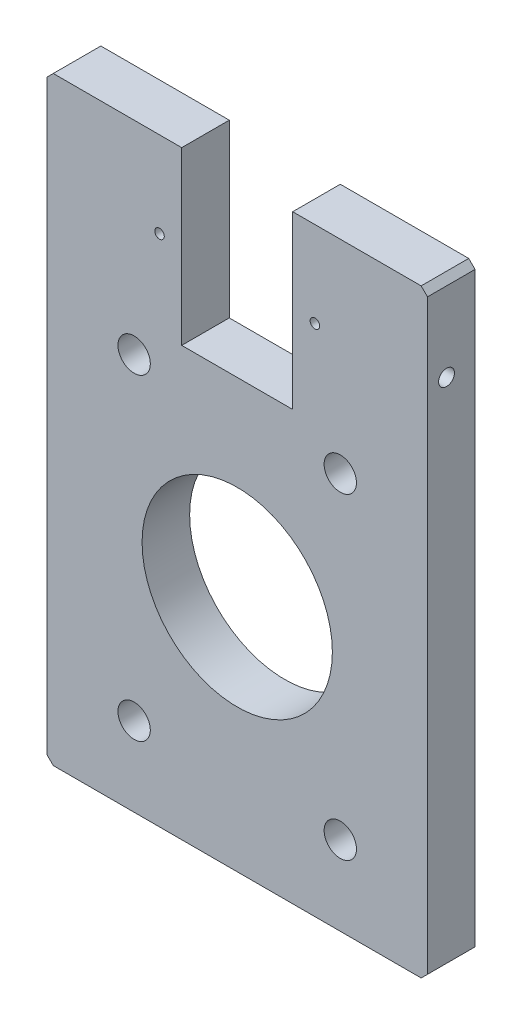
SolidWorks part; units mm, degrees
material "1023 碳钢板 (SS)"
ref_plane "Front Plane" through (0, 0, 0) normal (0, 0, 1) x (1, 0, 0)
ref_plane "Top Plane" through (0, 0, 0) normal (0, 1, 0) x (1, 0, 0)
ref_plane "Right Plane" through (0, 0, 0) normal (1, 0, 0) x (0, 0, -1)
sketch "Sketch1" plane through (0, 0, 0) normal (0, 0, 1) x (1, 0, 0)
  line L0 (17.5, 94.5) -> (58, 94.5)
  line L1 (-58, 94.5) -> (-17.5, 94.5)
  line L2 (-60, 92.5) -> (-60, -92.5)
  line L3 (-58, -94.5) -> (58, -94.5)
  line L4 (60, 92.5) -> (60, -92.5)
  line L5 (-60, 94.5) -> (60, -94.5) construction
  line L6 (-60, -94.5) -> (60, 94.5) construction
  line L8 (-17.5, 94.5) -> (-17.5, 40.5)
  line L9 (-17.5, 40.5) -> (17.5, 40.5)
  line L10 (17.5, 94.5) -> (17.5, 40.5)
  line L11 (-17.5, 148.5) -> (17.5, 40.5) construction
  line L12 (-17.5, 40.5) -> (17.5, 148.5) construction
  line L13 (-60, 92.5) -> (-58, 94.5)
  line L14 (58, 94.5) -> (60, 92.5)
  line L15 (-60, -92.5) -> (-58, -94.5)
  line L16 (58, -94.5) -> (60, -92.5)
  circle A0 centre (-32.5, -69.5) radius 5.1
  circle A1 centre (-32.5, 30.5) radius 5.1
  circle A2 centre (32.5, 30.5) radius 5.1
  circle A3 centre (32.5, -69.5) radius 5.1
  point P0 (0, 0)
  point P6 (0, 94.5)
  point P23 (0, -94.5)
  dimension "D13" = 32.5
  dimension "D15" = 10.2
  dimension "D16" = 65
  dimension "D1" = 120
  dimension "D2" = 189
  dimension "D3" = 35
  dimension "D4" = 108
  dimension "D5" = 2
  dimension "D6" = 45
  dimension "D7" = 2
  dimension "D8" = 45
  dimension "D9" = 2
  dimension "D10" = 45
  dimension "D11" = 2
  dimension "D12" = 45
  dimension "D14" = 25
  dimension "D17" = 100
  dimension "D18" = 100
  dimension "D19" = 65
extrude "Boss-Extrude1" add sketch "Sketch1" along normal blind 15
hole_wizard "Size mm dowel hole 1" positions "3DSketch6" profile "Sketch20" hole size "Ø3.0" standard "IS"
sketch3d "3DSketch6"
  point P0 (60, 67.5, 9)
  dimension "D1" = 9
  dimension "D2" = 27
sketch "Sketch20" plane through (60, 67.5, 9) normal (0, 1, 0) x (0, 0, -1)
  line L0 (0, 0) -> (0, 40)
  line L1 (0, 40) -> (1.5, 39.0987)
  line L2 (1.5, 39.0987) -> (1.5, 0)
  line L5 (1.5, 0) -> (0, 0)
  line L10 (0, 40) -> (-1.5, 39.0987) construction
  line L11 (0, -6.35) -> (0, 107.95) construction
  dimension "孔直径" = 3
  dimension "孔深度" = 40
  dimension "导头角度" = 118
hole_wizard "Size mm dowel hole 2" positions "3DSketch7" profile "Sketch21" hole size "Ø3.0" standard "IS"
sketch3d "3DSketch7"
  point P0 (-60, 67.5, 9)
  dimension "D1" = 27
  dimension "D2" = 9
sketch "Sketch21" plane through (-60, 67.5, 9) normal (0, 1, 0) x (0, 0, 1)
  line L0 (0, 0) -> (0, 40.9013)
  line L1 (0, 40.9013) -> (1.5, 40)
  line L2 (1.5, 40) -> (1.5, 0)
  line L5 (1.5, 0) -> (0, 0)
  line L10 (0, 40.9013) -> (-1.5, 40) construction
  line L11 (0, -6.35) -> (0, 107.95) construction
  dimension "孔直径" = 3
  dimension "孔深度" = 40
  dimension "导头角度" = 118
hole_wizard "M6 Tapped Hole1" positions "3DSketch8" profile "Sketch22" tap size "M6" standard "IS"
sketch3d "3DSketch8"
  line L0 (-20, 67.5, 9) -> (-60, 67.5, 9) construction
  circle A0 centre (20.9013, 67.5, 9) radius 1.5 construction
  point P0 (20.9013, 67.5, 9)
  point P4 (22.4013, 67.5, 9)
  point P5 (-60, 67.5, 9)
sketch "Sketch22" plane through (-60, 67.5, 9) normal (0, 1, 0) x (0, 0, 1)
  line L0 (0, 0) -> (0, 18.5022)
  line L1 (0, 18.5022) -> (2.5, 17)
  line L2 (2.5, 17) -> (2.5, 0)
  line L5 (2.5, 0) -> (0, 0)
  line L10 (0, 18.5022) -> (-2.5, 17) construction
  line L11 (0, -6.35) -> (0, 107.95) construction
  dimension "螺纹孔钻头直径" = 5
  dimension "螺纹孔钻头深度" = 17
  dimension "导头角度" = 118
cosmetic thread "Hole thread 5" parameters "D1"=12, "D2"=6
hole_wizard "M6 Tapped Hole2" positions "3DSketch9" profile "Sketch23" tap size "M6" standard "IS"
sketch3d "3DSketch9"
  line L0 (20.9013, 67.5, 9) -> (60, 67.5, 9) construction
  point P0 (60, 67.5, 9)
sketch "Sketch23" plane through (60, 67.5, 9) normal (0, 1, 0) x (0, 0, -1)
  line L0 (0, 0) -> (0, 18.5022)
  line L1 (0, 18.5022) -> (2.5, 17)
  line L2 (2.5, 17) -> (2.5, 0)
  line L5 (2.5, 0) -> (0, 0)
  line L10 (0, 18.5022) -> (-2.5, 17) construction
  line L11 (0, -6.35) -> (0, 107.95) construction
  dimension "螺纹孔钻头直径" = 5
  dimension "螺纹孔钻头深度" = 17
  dimension "导头角度" = 118
cosmetic thread "Hole thread 6" parameters "D1"=12, "D2"=6
hole_wizard "M12 Tapped Hole1" positions "3DSketch10" profile "Sketch25" tap size "M12" standard "IS" end condition through all
sketch3d "3DSketch10"
  line L0 (-32.5, 30.5, 15) -> (-32.5, 30.5, 0) construction
  line L1 (32.5, 30.5, 15) -> (32.5, 30.5, 0) construction
  line L2 (32.5, -69.5, 15) -> (32.5, -69.5, 0) construction
  line L3 (-32.5, -69.5, 15) -> (-32.5, -69.5, 0) construction
  point P0 (-32.5, 30.5, 15)
  point P4 (32.5, 30.5, 15)
  point P8 (32.5, -69.5, 15)
  point P12 (-32.5, -69.5, 15)
sketch "Sketch25" plane through (-32.5, 30.5, 15) normal (1, 0, 0) x (0, -1, 0)
  line L0 (0, 0) -> (0, 15)
  line L1 (0, 15) -> (5.1, 15)
  line L2 (5.1, 15) -> (5.1, 0)
  line L5 (5.1, 0) -> (0, 0)
  line L11 (0, -6.35) -> (0, 107.95) construction
  dimension "通孔螺纹孔钻头直径" = 10.2
  dimension "通孔螺纹孔钻头深度" = 15
cosmetic thread "Hole thread 7" parameters "D2"=12
cosmetic thread "Hole thread 8" parameters "D2"=12
cosmetic thread "Hole thread 9" parameters "D2"=12
cosmetic thread "Hole thread 10" parameters "D2"=12
sketch "Sketch26" plane through (0, 0, 15) normal (0, 0, 1) x (1, 0, 0)
  line L0 (58, 94.5) -> (17.5, 94.5) construction
  circle A0 centre (0, -19.5) radius 30
  dimension "D1" = 114
extrude "Cut-Extrude8" cut sketch "Sketch26" against normal blind 20
hole_wizard "Size mm dowel hole 3" positions "3DSketch11" profile "Sketch27" hole size "Ø3.0" standard "IS"
sketch3d "3DSketch11"
  line L0 (-17.5, 94.5, 15) -> (-58, 94.5, 15) construction
  line L1 (-17.5, 40.5, 15) -> (-17.5, 94.5, 15) construction
  line L2 (17.5, 94.5, 15) -> (17.5, 40.5, 15) construction
  line L3 (58, 94.5, 15) -> (17.5, 94.5, 15) construction
  point P0 (-24.5, 67.5, 15)
  point P2 (24.5, 67.5, 15)
  dimension "D1" = 27
  dimension "D2" = 7
  dimension "D3" = 7
  dimension "D4" = 27
sketch "Sketch27" plane through (-24.5, 67.5, 15) normal (1, 0, 0) x (0, -1, 0)
  line L0 (0, 0) -> (0, 20.6513)
  line L1 (0, 20.6513) -> (1.5, 19.75)
  line L2 (1.5, 19.75) -> (1.5, 0)
  line L5 (1.5, 0) -> (0, 0)
  line L10 (0, 20.6513) -> (-1.5, 19.75) construction
  line L11 (0, -6.35) -> (0, 107.95) construction
  dimension "孔直径" = 3
  dimension "孔深度" = 19.75
  dimension "导头角度" = 118
sketch "Sketch28" plane through (0, 0, 0) normal (0, 0, -1) x (-1, 0, 0)
  circle A0 centre (24.5, 67.5) radius 1.5 construction
  circle A1 centre (-24.5, 67.5) radius 1.5 construction
  circle A2 centre (24.5, 67.5) radius 1.5
  circle A3 centre (-24.5, 67.5) radius 1.5
extrude "Boss-Extrude2" add sketch "Sketch28" against normal blind 7 separate body
